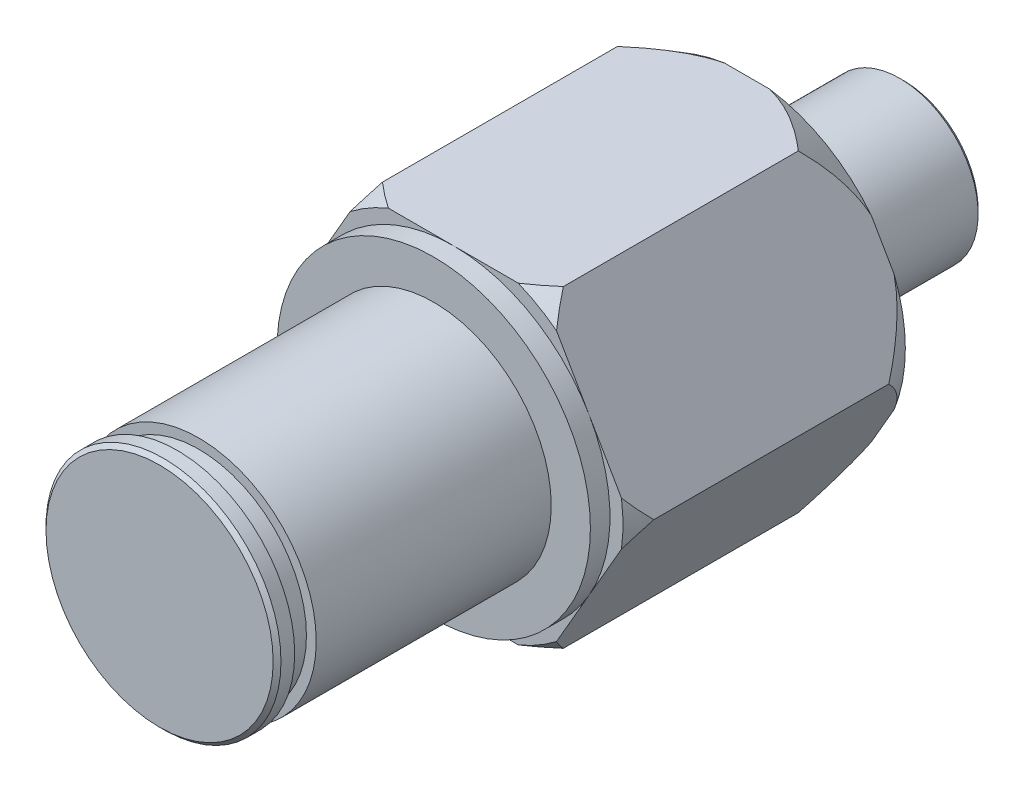
SolidWorks part; units mm, degrees
material "S45C"
ref_plane "Front Plane" through (0, 0, 0) normal (0, 0, 1) x (1, 0, 0)
ref_plane "Top Plane" through (0, 0, 0) normal (0, 1, 0) x (1, 0, 0)
ref_plane "Right Plane" through (0, 0, 0) normal (1, 0, 0) x (0, 0, -1)
sketch "Sketch1" plane through (0, 0, 0) normal (0, 0, 1) x (1, 0, 0)
  circle A0 centre (0, 50) radius 12.5
  dimension "D1" = 25
extrude "Boss-Extrude1" add sketch "Sketch1" along normal blind 30
sketch "Sketch2" plane through (0, 0, 0) normal (0, 0, -1) x (-1, 0, 0)
  line L1 (-4.6188, 42) -> (4.6188, 42)
  line L2 (4.6188, 42) -> (9.2376, 50)
  line L3 (9.2376, 50) -> (4.6188, 58)
  line L4 (4.6188, 58) -> (-4.6188, 58)
  line L5 (-4.6188, 58) -> (-9.2376, 50)
  line L6 (-9.2376, 50) -> (-4.6188, 42)
  circle A0 centre (0, 50) radius 8 construction
  dimension "D1" = 16
extrude "Cut-Extrude1" cut sketch "Sketch2" against normal blind 15 flip side to cut
sketch "Sketch3" plane through (0, 0, 15) normal (0, 0, -1) x (-1, 0, 0)
  circle A0 centre (0, 50) radius 8
  dimension "D1" = 16
extrude "Cut-Extrude2" cut sketch "Sketch3" against normal through all flip side to cut
sketch "Sketch4" plane through (0, 0, 0) normal (0, 0, -1) x (-1, 0, 0)
  circle A0 centre (0, 50) radius 4
  circle A1 centre (0, 50) radius 8 construction
  dimension "D1" = 8
extrude "Boss-Extrude2" add sketch "Sketch4" along normal blind 8
cosmetic thread "Cosmetic Thread1" parameters "D1"=10, "D2"=6.647
sketch "Sketch5" plane through (0, 0, 0) normal (0, 0, -1) x (-1, 0, 0)
  circle A0 centre (0, 50) radius 3.25
  dimension "D1" = 6.5
extrude "Cut-Extrude3" cut sketch "Sketch5" along normal blind 1.5 flip side to cut
sketch "Sketch6" plane through (0, 0, 30) normal (0, 0, 1) x (1, 0, 0)
  circle A0 centre (0, 50) radius 6
  dimension "D1" = 12
extrude "Cut-Extrude4" cut sketch "Sketch6" against normal blind 14 flip side to cut
ref_plane "Plane1" through (0, 0, 28) normal (0, 0, 1) x (1, 0, 0)
sketch "Sketch8" plane through (0, 0, 28) normal (0, 0, 1) x (1, 0, 0)
  circle A0 centre (0, 50) radius 5.5
  dimension "D1" = 11
extrude "Cut-Extrude5" cut sketch "Sketch8" along normal blind 1.1 flip side to cut
chamfer "Chamfer1" distance 0.2 angle 45 2 edges at (-4, 50, -8) (6, 50, 30)
ref_plane "Plane2" through (0, 50, 0) normal (0, 1, 0) x (1, 0, 0)
sketch "Sketch10" plane through (0, 50, 0) normal (0, 1, 0) x (1, 0, 0)
  line L0 (-9.2376, 0) -> (-9.2376, -2)
  line L1 (-9.2376, -15) -> (-9.2376, 0) construction
  line L2 (-9.2376, -2) -> (-8.0829, 0)
  line L3 (-9.2376, 0) -> (-4.6188, 0) construction
  line L4 (-8.0829, 0) -> (-9.2376, 0)
  line L5 (-9.2376, -15) -> (-9.2376, -14)
  line L6 (-9.2376, -14) -> (-8.6603, -15)
  line L7 (-9.2376, -15) -> (-6.9282, -15) construction
  line L8 (-8.6603, -15) -> (-9.2376, -15)
  line L9 (0, 8) -> (0, -26.0696) construction
  line L10 (3.8, 8) -> (-3.8, 8) construction
  dimension "D1" = 60
  dimension "D2" = 2
  dimension "D3" = 1
  dimension "D4" = 60
revolve "Cut-Revolve1" cut sketch "Sketch10" angle 360 about L9
